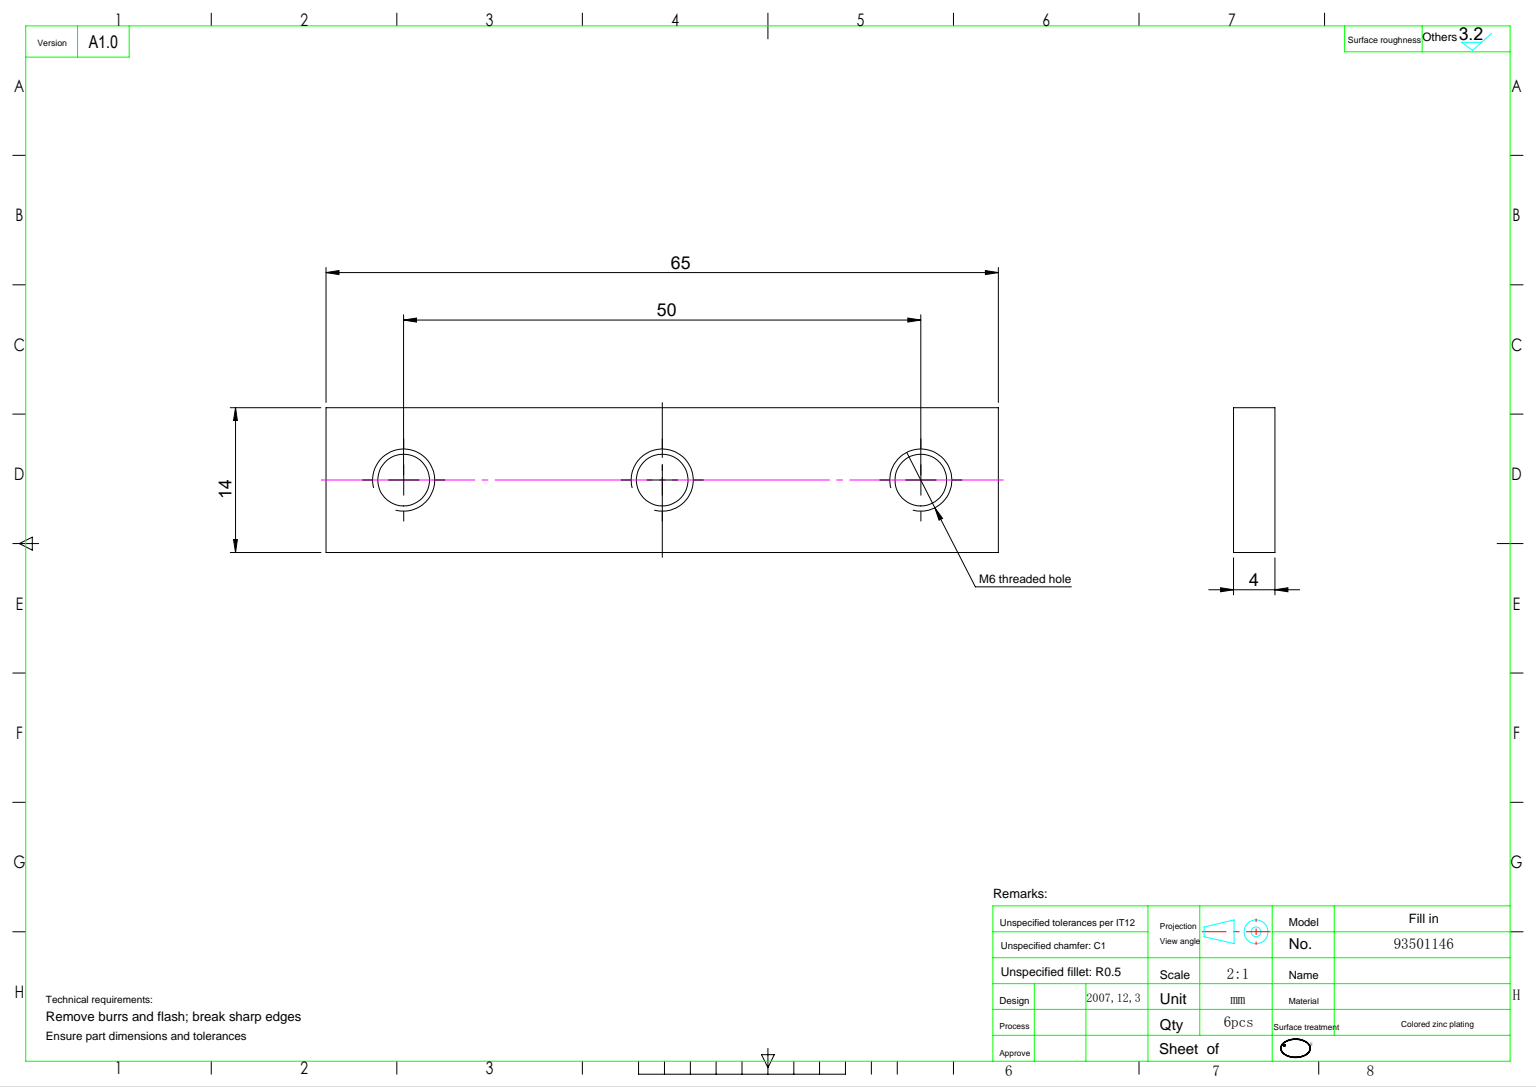
SolidWorks part; units mm, degrees
ref_plane "前视基准面" through (0, 0, 0) normal (0, 0, 1) x (1, 0, 0)
ref_plane "上视基准面" through (0, 0, 0) normal (0, 1, 0) x (1, 0, 0)
ref_plane "右视基准面" through (0, 0, 0) normal (1, 0, 0) x (0, 0, -1)
sketch "草图2" plane through (0, 0, 0) normal (0, 1, 0) x (1, 0, 0)
  line L1 (-32.5, 7) -> (32.5, 7)
  line L2 (-32.5, 7) -> (-32.5, -7)
  line L3 (-32.5, -7) -> (32.5, -7)
  line L4 (32.5, 7) -> (32.5, -7)
  line L5 (-32.5, 7) -> (32.5, -7) construction
  line L6 (-32.5, -7) -> (32.5, 7) construction
  point P0 (0, 0)
  dimension "D1" = 65
  dimension "D2" = 14
extrude "凸台-拉伸1" add sketch "草图2" along normal mid plane 4 separate body
hole_wizard "M6 螺纹孔1" positions "草图3" profile "草图4" tap size "M6" standard "GB" end condition through all
sketch "草图3" plane through (0, 2, 0) normal (0, 1, 0) x (1, 0, 0)
  line L0 (0, 0) -> (0, 12.5031) construction
  point P0 (-25, 0)
  point P2 (0, 0)
  point P12 (25, 0)
  dimension "D1" = 50
sketch "草图4" plane through (-25, 2, 0) normal (1, 0, 0) x (0, 0, 1)
  line L0 (0, 0) -> (0, 4)
  line L1 (0, 4) -> (2.5, 4)
  line L2 (2.5, 4) -> (2.5, 0)
  line L5 (2.5, 0) -> (0, 0)
  line L11 (0, -6.35) -> (0, 107.95) construction
  dimension "通孔螺纹孔钻头直径" = 5
  dimension "通孔螺纹孔钻头深度" = 4
cosmetic thread "孔螺蚊线1" parameters "D2"=6
cosmetic thread "孔螺蚊线2" parameters "D2"=6
cosmetic thread "孔螺蚊线3" parameters "D2"=6
